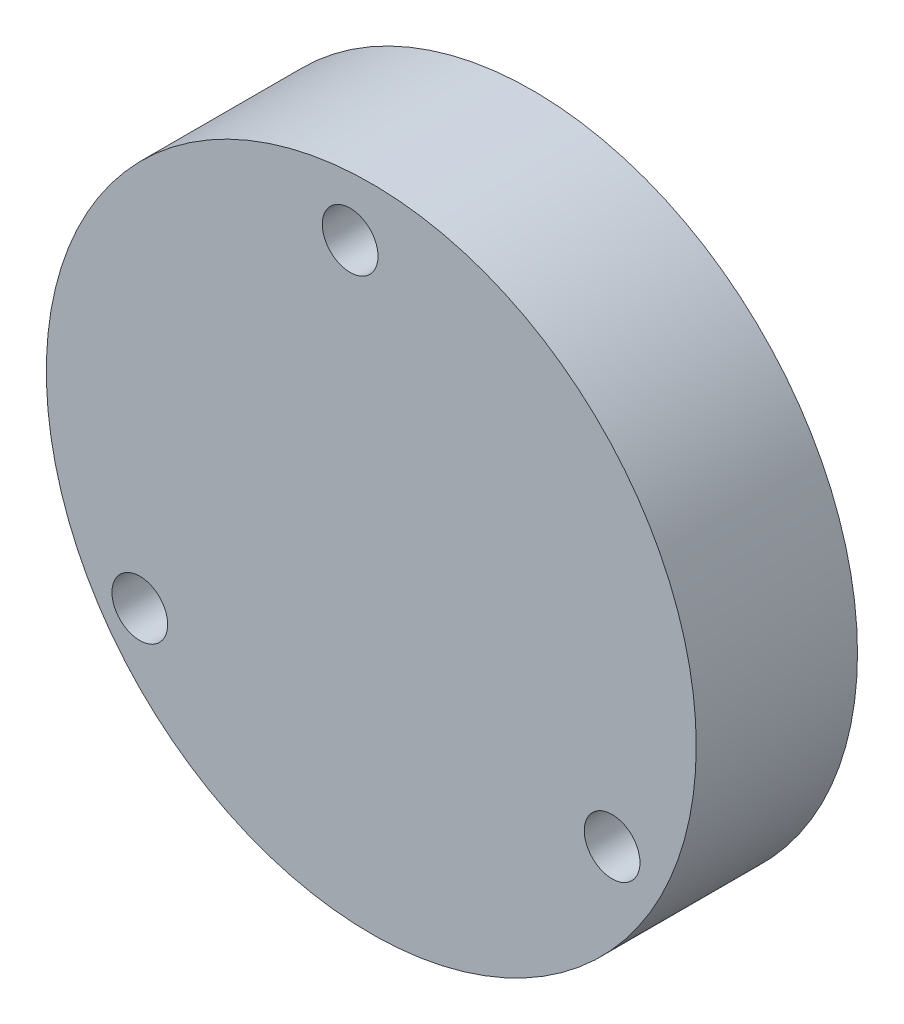
from build123d import *

# Parameters (mm, degrees)
MODEL_R             = 30.226848254
MODEL_R_2           = 2.590872707
BOSS_EXTRUDE1_DEPTH = 15


with BuildPart() as part:
    # Model → Boss-Extrude1 (new body)
    with BuildSketch(Plane.XY):
        with Locations((-14.795552969, -17.915164858)):
            Circle(MODEL_R)
        with Locations((-16.760867787, 6.745900605)):
            Circle(MODEL_R_2, mode=Mode.SUBTRACT)
        with Locations((-36.327028146, -32.68664647)):
            Circle(MODEL_R_2, mode=Mode.SUBTRACT)
        with Locations((7.605639537, -29.915164858)):
            Circle(MODEL_R_2, mode=Mode.SUBTRACT)
    extrude(amount=BOSS_EXTRUDE1_DEPTH)


solid = part.part
